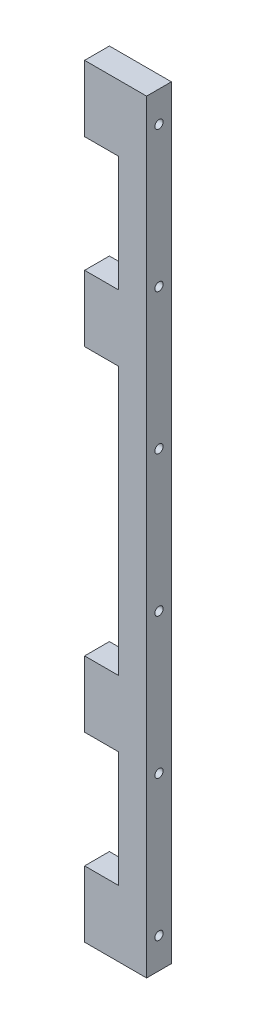
from build123d import *

# Parameters (mm, degrees)
EXTRUDE_1_DEPTH        = 15
CHAMFER_1_SIZE         = 3
HOLE_WIZARD_M6_1_D     = 5
HOLE_WIZARD_M6_1_DEPTH = 17
HOLE_WIZARD_M6_1_TIP   = 1.502151548


with BuildPart() as part:
    # 草图1 → 凸台-拉伸1 (new body)
    with BuildSketch(Plane.XY):
        Polygon((0, 462), (0, 422), (23.5, 422), (23.5, 352), (0, 352), (0, 312), (23.5, 312), (23.5, 150), (0, 150), (0, 110), (23.5, 110), (23.5, 40), (0, 40), (0, 0), (40.5, 0), (40.5, 462), align=None)
    extrude(amount=EXTRUDE_1_DEPTH)

    # 倒角1
    chamfer_1_edges = [part.edges().sort_by_distance(p)[0] for p in [
        (0, 20, 15),
        (0, 110, 7.5),
        (0, 150, 7.5),
        (0, 312, 7.5),
        (0, 352, 7.5),
        (0, 422, 7.5),
        (0, 462, 7.5),
        (0, 0, 7.5),
        (0, 40, 7.5),
        (0, 442, 15),
        (0, 332, 15),
        (0, 130, 15),
    ]]
    chamfer(chamfer_1_edges, length=CHAMFER_1_SIZE)

    # M6 螺纹孔1
    with Locations(Plane(origin=(40.5, 0, 0), x_dir=(0, 0, -1), z_dir=(1, 0, 0))):
        with Locations((-7.5, 443.5), (-7.5, 358.5), (-7.5, 273.5), (-7.5, 188.5), (-7.5, 103.5), (-7.5, 18.5)):
            Hole(HOLE_WIZARD_M6_1_D / 2, depth=HOLE_WIZARD_M6_1_DEPTH)
            with Locations((0, 0, -(HOLE_WIZARD_M6_1_DEPTH + HOLE_WIZARD_M6_1_TIP / 2))):  # 118° drill point
                Cone(0, HOLE_WIZARD_M6_1_D / 2, HOLE_WIZARD_M6_1_TIP, mode=Mode.SUBTRACT)


solid = part.part
